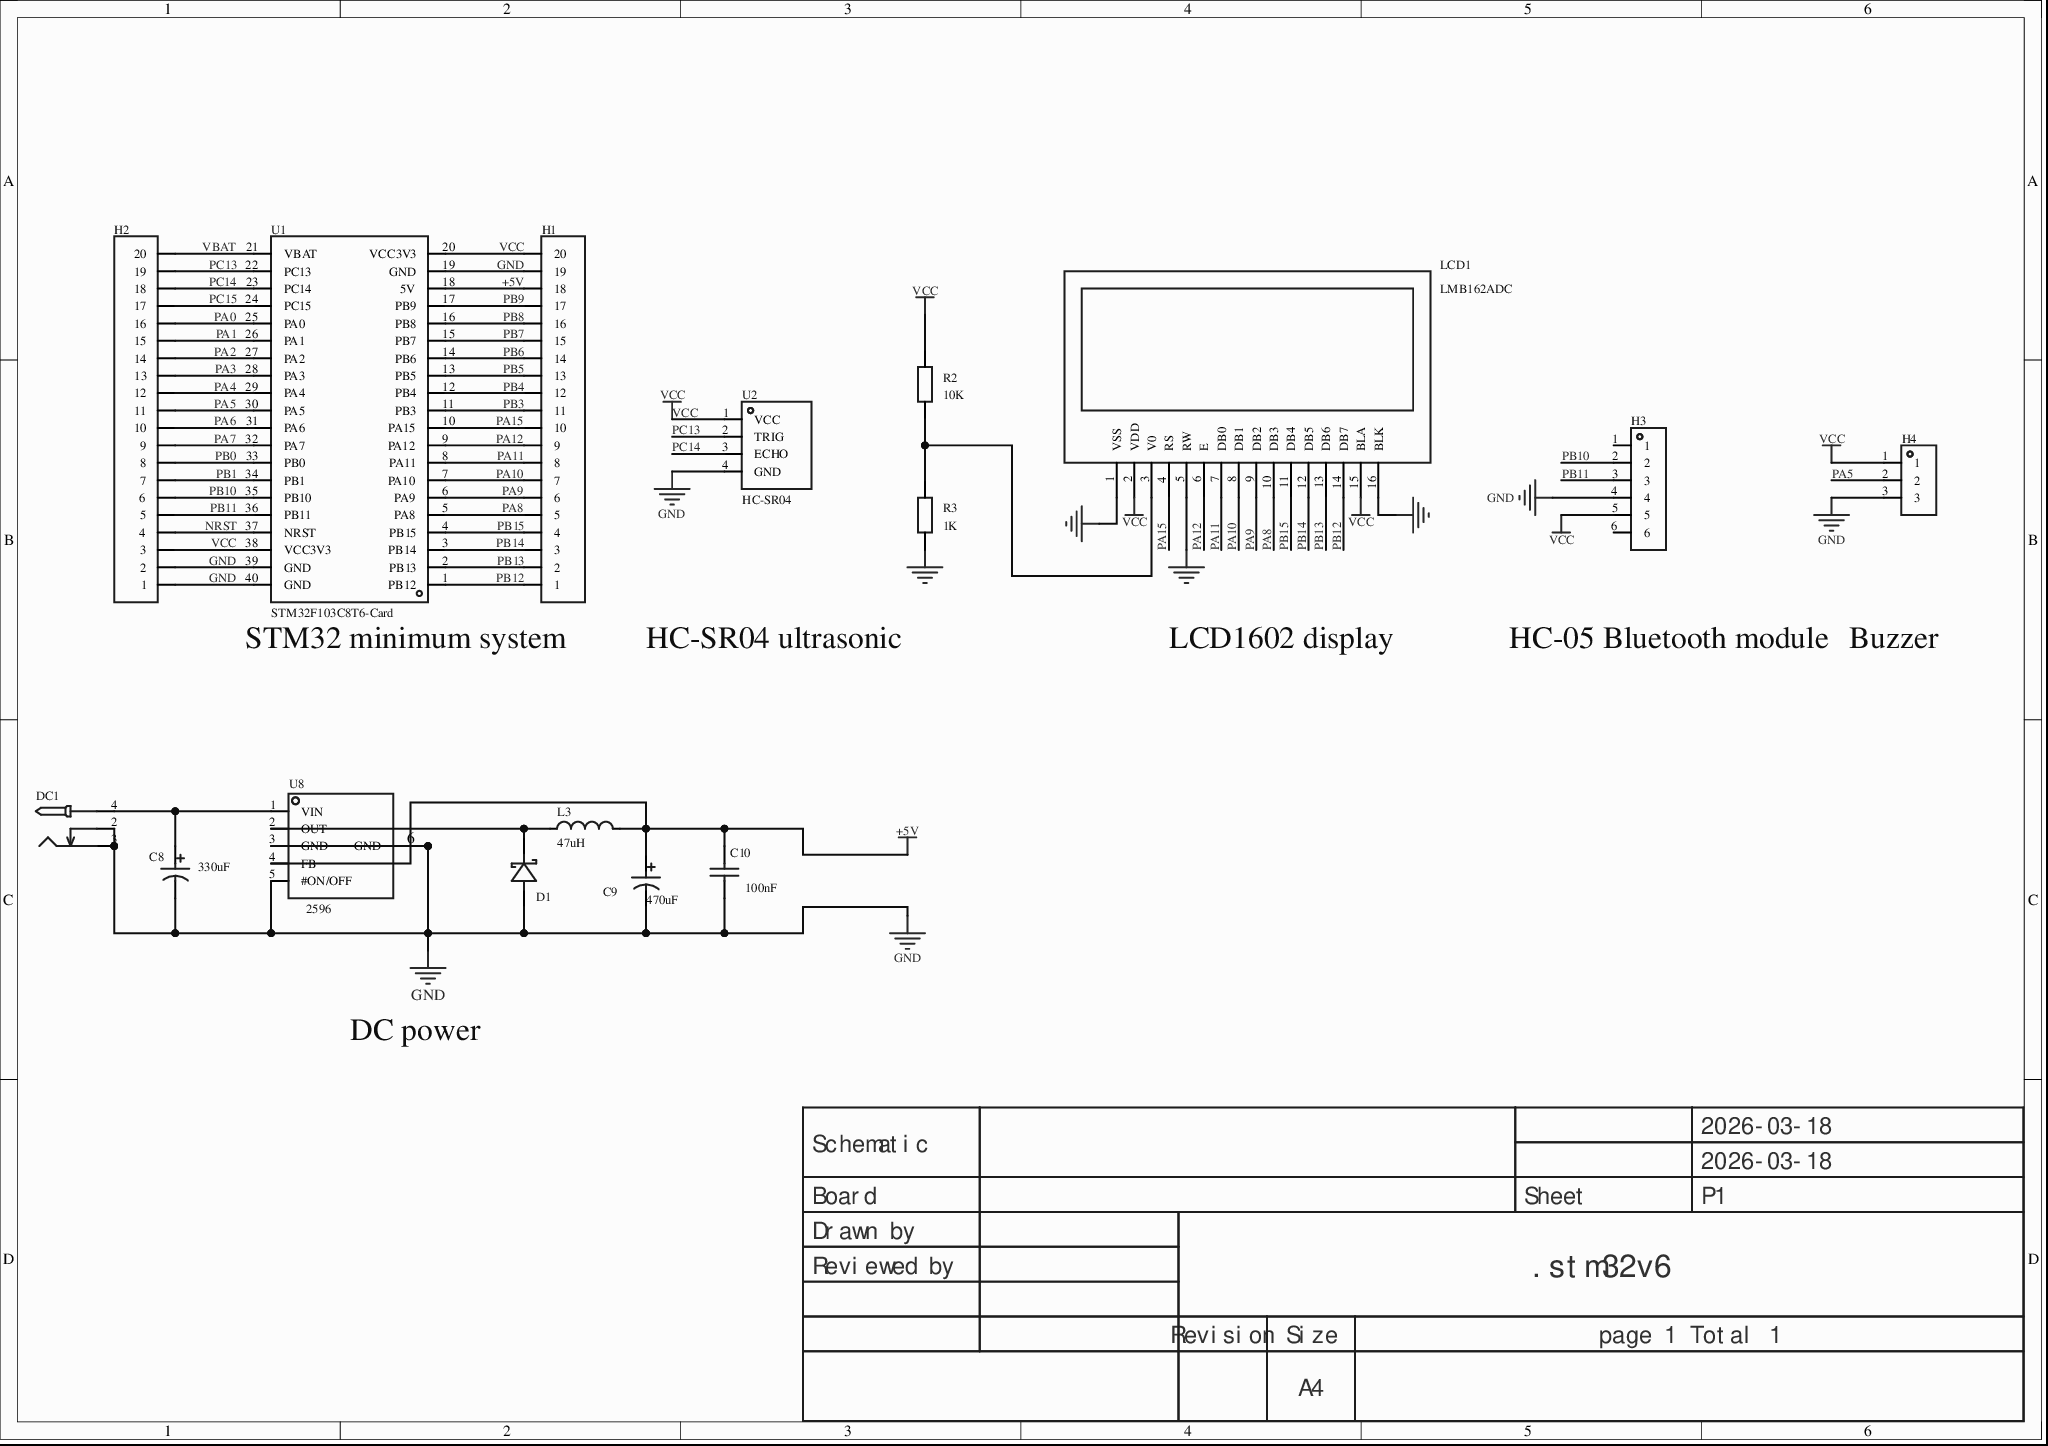
[diagram p0: MISC89129-3.schdoc]
# Altium project MISC89129-2.PrjPcb
1 sheet, 16 parts. Net scope: global (net labels, ports and power ports of the same name join across sheets).
Board file: MISC89129.pcbdoc

## Sheet MISC89129-3.schdoc
size 297 x 209 mm; Version: V1.0; @Project Name: MISC89129; @Page Count: 1; @Update Date: 2026-03-18; @Create Date: 2026-03-18; @Schematic Name: MISC89129; @Page No: 1; @Create Time: 23:22:16; @Update Time: 17:32:40; @Board Name: MISC89129

### Parts
C8  value 330uF  [CAP-SMD_BD8.0-L8.3-W8.3-RD]
C9  value 470uF  [CAP-SMD_BD8.0-L8.3-W8.3-RD]
C10  value 100nF  [C0805]
D1  (no value)  [SMA_L4.3-W2.6-LS5.2-RD]
DC1  (no value)  [DC-2.0]
H1  (no value)  [HDR-TH_20P-P2.54-V-F]
H2  (no value)  [HDR-TH_20P-P2.54-V-F]
H3  (no value)  [HDR-TH_6P-P2.54-V-F]
H4  (no value)  [HDR-TH_3P-P2.54-V-F]
L3  value 47uH  [IND-SMD_L7.0-W6.6]
LCD1  LMB162ADC  [LCD1602]
R2  10K  [R0805]
R3  1K  [R0805]
U1  STM32F103C8T6-Card  [CONN-TH_L53.3-W22.9_STM32F103C8T6-CARD]
U2  HC-SR04  [TH_HC-SR04V]
U8  LM2596S-5.0  [TO-263-5_L10.2-W8.9-P1.70-BR]  (value not drawn)

### Nets
+5V: C9.1 C10.1 H1.18 L3.2 U1.18(5V) U8.4(FB)
GND: C8.2 C9.2 C10.2 D1.2(A) DC1.2 DC1.3 H1.19 H2.1 H2.2 H3.4 H4.3 LCD1.1(VSS) LCD1.5(RW) LCD1.16(BLK) R3.1 U1.19(GND) U1.39(GND) U1.40(GND) U2.4(GND) U8.3(GND) U8.5(#ON/OFF) U8.6(GND)
VCC: H1.20 H2.3 H3.5 H4.1 LCD1.2(VDD) LCD1.15(BLA) R2.2 U1.20(VCC3V3) U1.38(VCC3V3) U2.1(VCC)
NRST: H2.4 U1.37(NRST)
PA0: H2.16 U1.25(PA0)
PA1: H2.15 U1.26(PA1)
PA2: H2.14 U1.27(PA2)
PA3: H2.13 U1.28(PA3)
PA4: H2.12 U1.29(PA4)
PA5: H2.11 H4.2 U1.30(PA5)
PA6: H2.10 U1.31(PA6)
PA7: H2.9 U1.32(PA7)
PA8: H1.5 LCD1.10(DB3) U1.5(PA8)
PA9: H1.6 LCD1.9(DB2) U1.6(PA9)
PA10: H1.7 LCD1.8(DB1) U1.7(PA10)
PA11: H1.8 LCD1.7(DB0) U1.8(PA11)
PA12: H1.9 LCD1.6(E) U1.9(PA12)
PA15: H1.10 LCD1.4(RS) U1.10(PA15)
PB0: H2.8 U1.33(PB0)
PB1: H2.7 U1.34(PB1)
PB3: H1.11 U1.11(PB3)
PB4: H1.12 U1.12(PB4)
PB5: H1.13 U1.13(PB5)
PB6: H1.14 U1.14(PB6)
PB7: H1.15 U1.15(PB7)
PB8: H1.16 U1.16(PB8)
PB9: H1.17 U1.17(PB9)
PB10: H2.6 H3.2 U1.35(PB10)
PB11: H2.5 H3.3 U1.36(PB11)
PB12: H1.1 LCD1.14(DB7) U1.1(PB12)
PB13: H1.2 LCD1.13(DB6) U1.2(PB13)
PB14: H1.3 LCD1.12(DB5) U1.3(PB14)
PB15: H1.4 LCD1.11(DB4) U1.4(PB15)
PC13: H2.19 U1.22(PC13) U2.2(TRIG)
PC14: H2.18 U1.23(PC14) U2.3(ECHO)
PC15: H2.17 U1.24(PC15)
VBAT: H2.20 U1.21(VBAT)
NetC8_1: C8.1 DC1.4 U8.1(VIN)
NetD1_1: D1.1(K) L3.1 U8.2(OUT)
NetLCD1_3: LCD1.3(V0) R2.1 R3.2

Not connected (* = marked no-connect by the designer): H3 1 6

### Notes on the sheet
- STM32 minimum system
- HC-SR04 ultrasonic
- LCD1602 display
- HC-05 Bluetooth module
- Buzzer
- DC power
- Labels drawn without touching a wire or pin: VCC
- 2026-03-18
- Schematic
- Board
- Sheet
- P1
- Drawn by
- Reviewed by
- .stm32v6
- Revision
- Size
- A4
- page 1 Total 1

### Library data of the parts
C8 C9 = CS1V221M-CRF10　: Capacitance: 220uF; tolerance: ±20%; rated voltage: 35V; capacitor body diameter: 8mm; body length: 10.5mm; ripple current: -; ESR: -; operating life: 2000hrs@105; operating temperature: -40~+105;; Manufacturer: ST(先科); Rated Voltage: 25V; 3D Model: b102f1362be24624a1b1334fec8dc7f4; 3D Model Transform: 354.33,326.81037,0,0,0,0,0,0,0; AddInBom: yes; Symbol: CS1V221M-CRF10; Device: CS1V221M-CRF10; Lifetime @ Temp: 2000hrs@105; Operating Temperature: -40~+105; Manufacturer Part: CS1V221M-CRF10; Supplier Footprint: SMD,8x10.5mm; JLCPCB Part Class: Extended Part; Datasheet: https://atta.szlcsc.com/upload/public/pdf/source/20170325/1490427945143.pdf; Supplier: LCSC; Tolerance: ±20%; φD: 8mm; L: 10.5mm; Ripple Current: -; Equivalent Series Resistance(ESR): -; ConvertToPcb: yes; FootprintName: CAP-SMD_BD8.0-L8.3-W8.3-RD; ModelName: CAP-SMD_BD8.0-L8.3-W8.3-RD
  C8: Supplier Part: C97814
C10 = CL21B104KBCNNNC: Capacitance: 100nF; tolerance: ±10%; rated voltage: 50V; temperature coefficient: X7R;; Manufacturer: SAMSUNG(三星); 3D Model: 1ba041120af144c991958decab20d241; 3D Model Transform: 78.74,51.181,0,0,0,0,0,0.0005,0; AddInBom: yes; ModelName: C0805_L2.0-W1.3-H1.3; Symbol: CL21B104KBCNNNC; Device: CL21B104KBCNNNC; LCSC Part Name: 100nF ±10% 50V; Supplier Part: C1711; Manufacturer Part: CL21B104KBCNNNC; Supplier Footprint: 0805; JLCPCB Part Class: Extended Part; Datasheet: https://atta.szlcsc.com/upload/public/pdf/source/20160103/1457707693305.pdf; Supplier: LCSC; Tolerance: ±10%; Voltage Rated: 50V; Temperature Coefficient: X7R; ConvertToPcb: yes; FootprintName: C0805
D1 = SS34_3: Manufacturer: TDD(台冠电子); Manufacturer Part: SS34; Symbol: SS34_C3032484; 3D Model: 7ed2c9d0a4a74bbdbba07ab4052caf5b; 3D Model Transform: 185.039,102.362,0,0,0,0,0,0,0; AddInBom: yes; Device: SS34_3; LCSC Part Name: SS34; Supplier Part: C3032484; Supplier Footprint: SMA; JLCPCB Part Class: Extended Part; Datasheet: https://atta.szlcsc.com/upload/public/pdf/source/20220622/9D70D0693761B542BF6F533590093AA5.pdf; Supplier: LCSC; ConvertToPcb: yes; FootprintName: SMA_L4.3-W2.6-LS5.2-RD; ModelName: SMA_L4.3-W2.6-LS5.2-RD
DC1 = DC-005_2.0: Symbol: DC power jack; ConvertToPcb: yes; ModelId: f5f20b8a2308479b936ba3c2698865bb0819f05c4eef4c71ace90d822a990e87; ModelName: DC-IN-TH_DC-5520-1; ModelTransform: 372.05,551.18,582.68,90,0,0,137.8,0,-149.61; Device: DC-005_2.0; AddInBom: yes; Supplier Footprint: 插件; FootprintName: DC-2.0
H1 H2 = HDR-F_2.54_1x20P: ConvertToPcb: yes; ModelId: db7015f7ad9d48b8a3b1188db02e3429; ModelName: HDR-F-2.54_1x20; ModelTransform: 1999.996,100,0,0,0,0,0,0,-118.11; Device: HDR-F_2.54_1x20P; Symbol: HDR-F_2.54_1x20P; AddInBom: yes; SupplierPart: C50984; Supplier Footprint: 插件; FootprintName: HDR-TH_20P-P2.54-V-F
H3 = HDR-F_2.54_1x6P: Symbol: Header-Female-2.54_1x6; ConvertToPcb: yes; ModelId: 0f5bcf94dcda47d085f24cdca1696fe9; ModelTransform: 619.684,94.488,0,0,0,0,0,0,-125.984; Device: HDR-F_2.54_1x6P; AddInBom: yes; SupplierPart: C40877; Supplier Footprint: 插件; FootprintName: HDR-TH_6P-P2.54-V-F; ModelName: HDR-TH_6P-P2.54-V-F
H4 = HDR-F_2.54_1x3P: Symbol: PM254V-11-03-H85; ConvertToPcb: yes; ModelId: f3b3cc5aae9641bf9e56fc160cef875b; ModelName: HDR2.54-F-LI-1X3P; ModelTransform: 299.9994,100,0,0,0,0,0,0,-118.11; Device: HDR-F_2.54_1x3P; AddInBom: yes; SupplierPart: C541850; Supplier Footprint: 插件; FootprintName: HDR-TH_3P-P2.54-V-F
L3 = CMLO0630H330MTT: Inductance: 33uH; tolerance: ±20%; DC resistance (DCR): 270mΩ;; Manufacturer: Cybermax(思博科技); 3D Model: 6860c29aec394a38a0f014af7f722a42; 3D Model Transform: 275.6,259.8,0,0,0,0,0,0,0; AddInBom: yes; ModelName: IND-SMD_L7.0-W6.6-H3.0; Symbol: CMLO0630H330MTT; Device: CMLO0630H330MTT; LCSC Part Name: 33uH ±20% 270mΩ; Manufacturer Part: CMLO0630H330MTT; Supplier Footprint: SMD; JLCPCB Part Class: Extended Part; Datasheet: https://atta.szlcsc.com/upload/public/pdf/source/20201124/C961478_55C23F293F63DC1D2CF3D7AB16D0E182.pdf; Supplier: LCSC; Tolerance: ±20%; DC Resistance (DCR): 270mΩ; ConvertToPcb: yes; FootprintName: IND-SMD_L7.0-W6.6
LCD1 = LMB162ADC: 16x2 character LCD module; 3D Model: f9d832f46a914cadb50fc4d4cefd2517; 3D Model Transform: 3149.6,1417.32,0,0,0,0,0,0,-118.11; AddInBom: yes; Symbol: LMB162ADC; Device: LMB162ADC; LCSC Part Name: LMB162ADC; Supplier Part: C9741; Manufacturer Part: LMB162ADC; Supplier Footprint: SIP; JLCPCB Part Class: Extended library; Supplier: LCSC; ConvertToPcb: yes; FootprintName: LCD1602; ModelName: LCD1602
R2 R3 = Res_0805: Symbol: Resistor; 3D Model: 37a81e68749a4138bd2dfa6897b24b85; 3D Model Transform: 78.74,51.181,0,0,0,0,0,-0.0005,0; ConvertToPcb: yes; ModelName: R0805_L2.0-W1.3-H0.6; Device: Res_0805; Supplier Footprint: 0805; AddInBom: yes; FootprintName: R0805
  R2: Value: 10K
  R3: Value: 1K
U1 = STM32F103C8T6-Card: AddInBom: yes; Symbol: STM32F103C8T6-CARD; Device: STM32F103C8T6-Card; LCSC Part Name: STM32F103C8T6-Card; SupplierPart: C9900077949; ManufacturerPart: STM32F103C8T6-Card; Supplier Footprint: 插件; Supplier: LCSC; ConvertToPcb: yes; FootprintName: CONN-TH_L53.3-W22.9_STM32F103C8T6-CARD
U2 = HC-SR04: Manufacturer: Universal Microelectronics; AddInBom: yes; Symbol: HC-SR04; Device: HC-SR04; LCSC Part Name: HC-SR04; SupplierPart: C19857336; ManufacturerPart: HC-SR04; Supplier Footprint: -; JLCPCB Part Class: Extended library; Datasheet: https://atta.szlcsc.com/upload/public/pdf/source/20240122/47B8E374E428935B7962A2189EF91AAC.pdf; Supplier: LCSC; ConvertToPcb: yes; FootprintName: TH_HC-SR04V
U8 = LM2596S-5.0_C347421: Function type: step-down; output type: fixed; input voltage: 40V; output voltage: 5V; output current (max): 3A;; Manufacturer: UMW(广东友台半导体); Symbol: LM2596-TO263; Add into BOM: yes; 3D Model: 4e421a816a7f4d57b8710832ddea550a; 3D Model Transform: 401.574,560.17797,0,90,0,0,-45.276,0,0; Synchronous Rectification: No; Number of Outputs: 1; Topology: Buck; Switching Frequency: 150kHz; ModelName: TO-263-5-5P_L10.2-W8.7-H4.5-LS14.4-P1.70; Device: LM2596S-5.0_C347421; Convert to PCB: yes; LCSC Part Name: 降压型 输入40V 输出5V 3A; Supplier Part: C347421; Manufacturer Part: LM2596S-5.0; Supplier Footprint: TO-263-5; JLCPCB Part Class: Extended Part; Datasheet: https://atta.szlcsc.com/upload/public/pdf/source/20211011/C7416AEF3194BD283261B8F2553C4145.pdf; Supplier: LCSC; Function: Step-down; Output Type: Fixed; Input Voltage: 40V; Output Voltage: 5V; Output Current (Max): 3A; Operating Temperature: -40℃~+125℃@(TA); FootprintName: TO-263-5_L10.2-W8.9-P1.70-BR